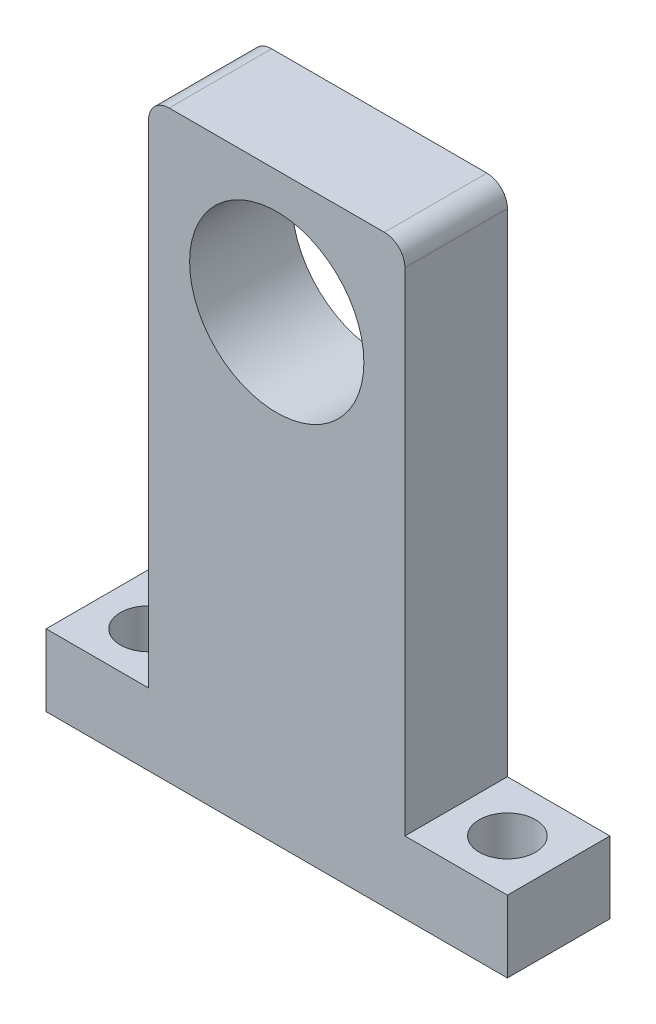
SolidWorks part; units mm, degrees
ref_plane "前视基准面" through (0, 0, 0) normal (0, 0, 1) x (1, 0, 0)
ref_plane "上视基准面" through (0, 0, 0) normal (0, 1, 0) x (1, 0, 0)
ref_plane "右视基准面" through (0, 0, 0) normal (1, 0, 0) x (0, 0, -1)
sketch "草图1" plane through (0, 0, 0) normal (0, 0, 1) x (1, 0, 0)
  line L0 (0, 0) -> (-22.5, 0)
  line L1 (-22.5, 0) -> (-22.5, 7)
  line L2 (-22.5, 7) -> (-12.5, 7)
  line L3 (-12.5, 7) -> (-12.5, 57)
  line L4 (-12.5, 57) -> (12.5, 57)
  line L5 (12.5, 57) -> (12.5, 7)
  line L6 (12.5, 7) -> (22.5, 7)
  line L7 (22.5, 7) -> (22.5, 0)
  line L8 (22.5, 0) -> (0, 0)
  circle A0 centre (0, 45) radius 8.5
  dimension "D3" = 17
  dimension "D1" = 10
  dimension "D2" = 7
  dimension "D4" = 12
  dimension "D5" = 45
  dimension "D6" = 25
extrude "凸台-拉伸1" add sketch "草图1" along normal mid plane 10
fillet "圆角1" radius 2 2 edges at (-12.5, 57, 0) (12.5, 57, 0)
sketch "草图2" plane through (0, 7, 0) normal (0, 1, 0) x (1, 0, 0)
  line L0 (-22.5, -5) -> (-22.5, 5) construction
  line L1 (22.5, -5) -> (22.5, 5) construction
  circle A0 centre (-17.5, 0) radius 2.75
  circle A1 centre (17.5, 0) radius 2.75
extrude "切除-拉伸1" cut sketch "草图2" against normal up to next
equation "\"D3@草图2\"=\"D2@草图2\""
